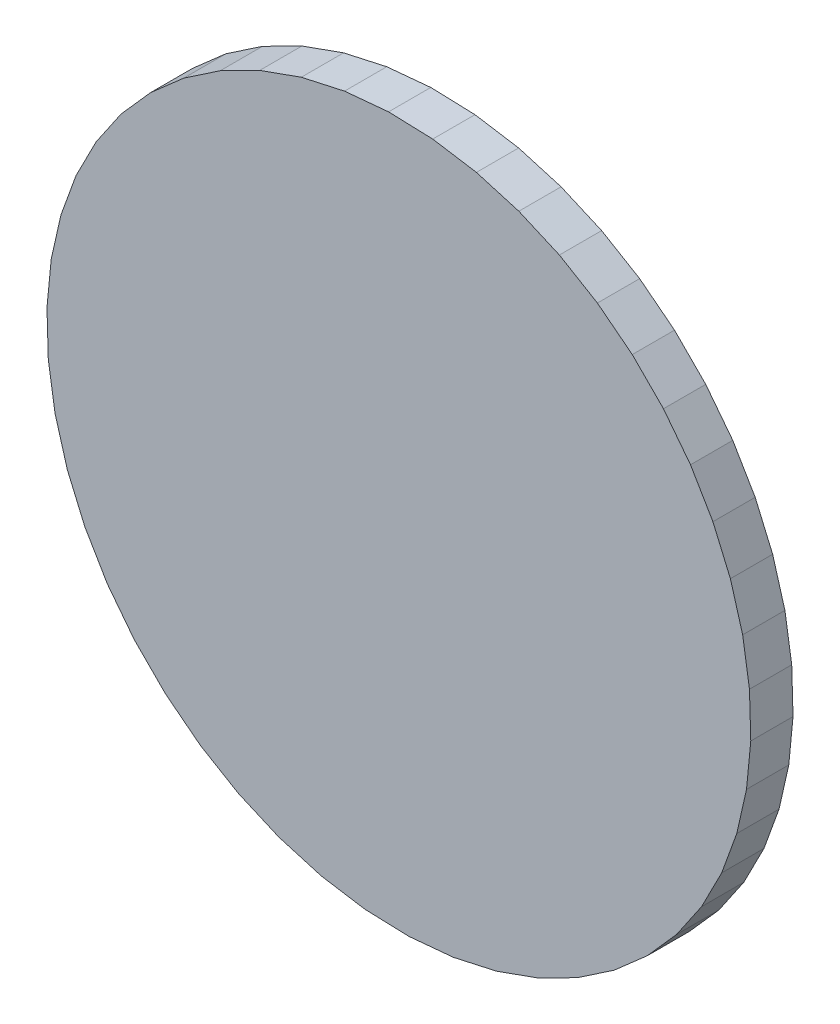
from build123d import *

# Parameters (mm, degrees)
BOSS_EXTRUDE1_DEPTH = 2.999998629


with BuildPart() as part:
    # Sketch1 → Boss-Extrude1 (new body)
    with BuildSketch(Plane(origin=(0, 0, 36.080602556), x_dir=(-1, 0, 0), z_dir=(0, 0, -1))):
        Polygon((24.985987693, 0.836887804), (24.684077129, 3.961863462), (23.992881179, 7.024358027), (22.923305631, 9.9760741), (21.492214873, 12.77046185), (19.722178578, 15.363452025), (17.641114071, 17.714152113), (15.281835571, 19.785488024), (12.681555003, 21.544793621), (9.8812785, 22.964326665), (6.925167516, 24.021700025), (3.85984336, 24.700235575), (0.733646855, 24.989232421), (-2.404119587, 24.884136394), (-5.503971595, 24.38659966), (-8.517022245, 23.504475132), (-11.395755224, 22.251669317), (-14.094769023, 20.647941157), (-16.57150127, 18.718581647), (-18.786890432, 16.49402082), (-20.705999807, 14.009339735), (-22.298563272, 11.303720996), (-23.539463058, 8.419836871), (-24.409133941, 5.403167102), (-24.893855676, 2.301285975), (-24.985987693, -0.836887804), (-24.684077129, -3.961863462), (-23.992881179, -7.024358027), (-22.923305631, -9.9760741), (-21.492214873, -12.77046185), (-19.722178578, -15.363452025), (-17.641114071, -17.714152113), (-15.281835571, -19.785488024), (-12.681555003, -21.544793621), (-9.8812785, -22.964326665), (-6.925167516, -24.021700025), (-3.85984336, -24.700235575), (-0.733646855, -24.989232421), (2.404119587, -24.884136394), (5.503971595, -24.38659966), (8.517022245, -23.504475132), (11.395755224, -22.251669317), (14.094769023, -20.647941157), (16.57150127, -18.718581647), (18.786890432, -16.49402082), (20.705999807, -14.009339735), (22.298563272, -11.303720996), (23.539463058, -8.419836871), (24.409133941, -5.403167102), (24.893855676, -2.301285975), align=None)
    extrude(amount=-BOSS_EXTRUDE1_DEPTH)


solid = part.part
